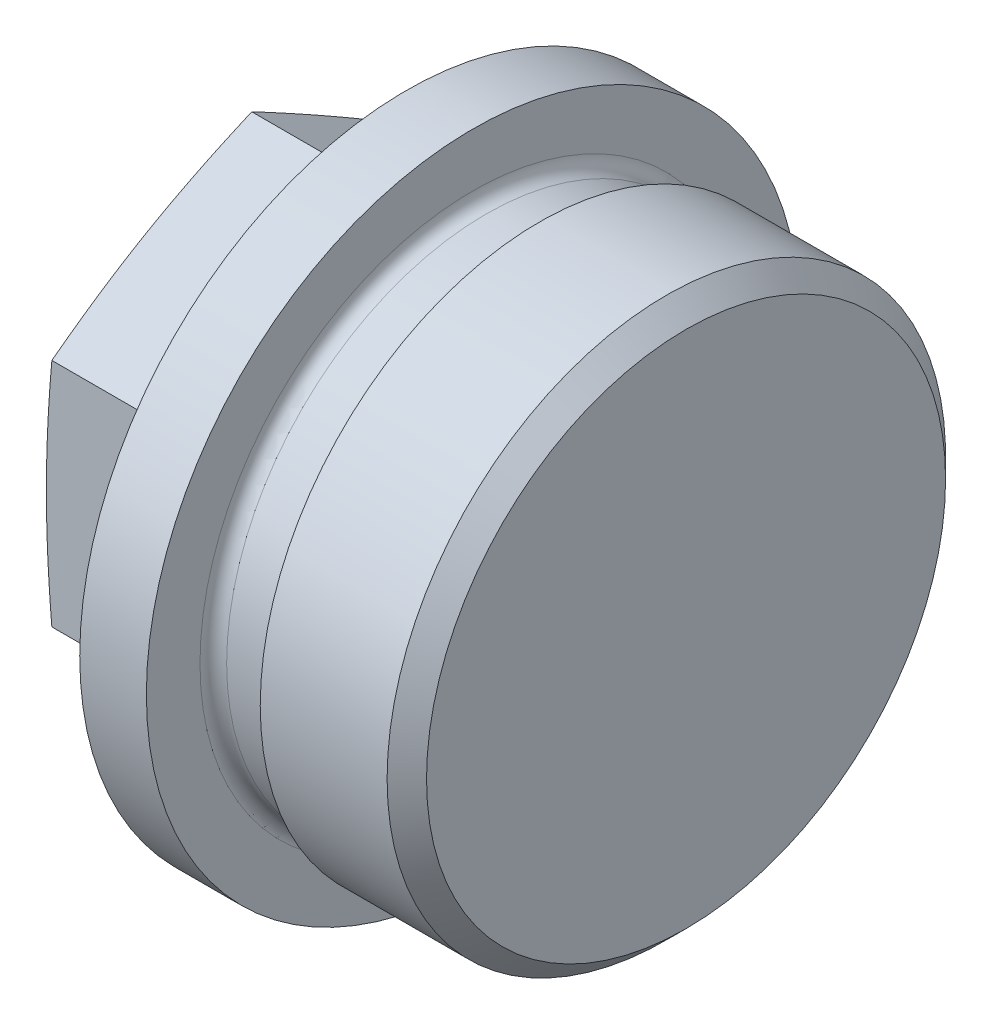
SolidWorks part; units mm, degrees
material "35钢"
ref_plane "Front Plane" through (0, 0, 0) normal (0, 0, 1) x (1, 0, 0)
ref_plane "Top Plane" through (0, 0, 0) normal (0, 1, 0) x (1, 0, 0)
ref_plane "Right Plane" through (0, 0, 0) normal (1, 0, 0) x (0, 0, -1)
sketch "Sketch1" plane through (0, 0, 0) normal (0, 0, 1) x (1, 0, 0)
  line L0 (0, 0) -> (33, 0) construction
  line L1 (33, 0) -> (33, 20.955) construction
  line L2 (33, 20.955) -> (22, 20.955) construction
  line L3 (22, 20.955) -> (22, 19.476)
  line L4 (22, 19.476) -> (17, 19.476)
  line L5 (17, 19.476) -> (17, 24.5)
  line L6 (17, 24.5) -> (12, 24.5)
  line L7 (12, 24.5) -> (12, 1.5)
  line L8 (12, 1.5) -> (0, 1.5)
  line L9 (0, 1.5) -> (0, 0)
  line L10 (0, 0) -> (33, 0)
  line L11 (31.521, 20.955) -> (33, 19.476)
  line L12 (22, 20.955) -> (31.521, 20.955)
  line L13 (33, 19.476) -> (33, 0)
  dimension "L" = 33
  dimension "b" = 5
  dimension "1" = 16
  dimension "d" = 41.91
  dimension "Do" = 49
  dimension "D6" = 3
  dimension "d1" = 38.952
  dimension "D8" = 45
revolve "Revolve1" add sketch "Sketch1" angle 360 about L0
sketch "Sketch2" plane through (0, 0, 0) normal (-1, 0, 0) x (0, 0, 1)
  line L1 (0, 17.3205) -> (-15, 8.6603)
  line L2 (-15, 8.6603) -> (-15, -8.6603)
  line L3 (-15, -8.6603) -> (0, -17.3205)
  line L4 (0, -17.3205) -> (15, -8.6603)
  line L5 (15, -8.6603) -> (15, 8.6603)
  line L6 (15, 8.6603) -> (0, 17.3205)
  circle A0 centre (0, 0) radius 15 construction
  dimension "s" = 30
extrude "Extrude1" add sketch "Sketch2" against normal up to surface (12 mm away) up to face at (12, 0, 1.5)
sketch "Sketch3" plane through (0, 0, 0) normal (-1, 0, 0) x (0, 0, 1)
  circle A0 centre (0, 0) radius 15 construction
  circle A1 centre (0, 0) radius 15
extrude "Cut-Extrude1" cut sketch "Sketch3" against normal blind 10 draft 80 flip side to cut
fillet "Fillet1" radius 1 2 edges at (22, 0, 19.476) (17, 0, 19.476)
